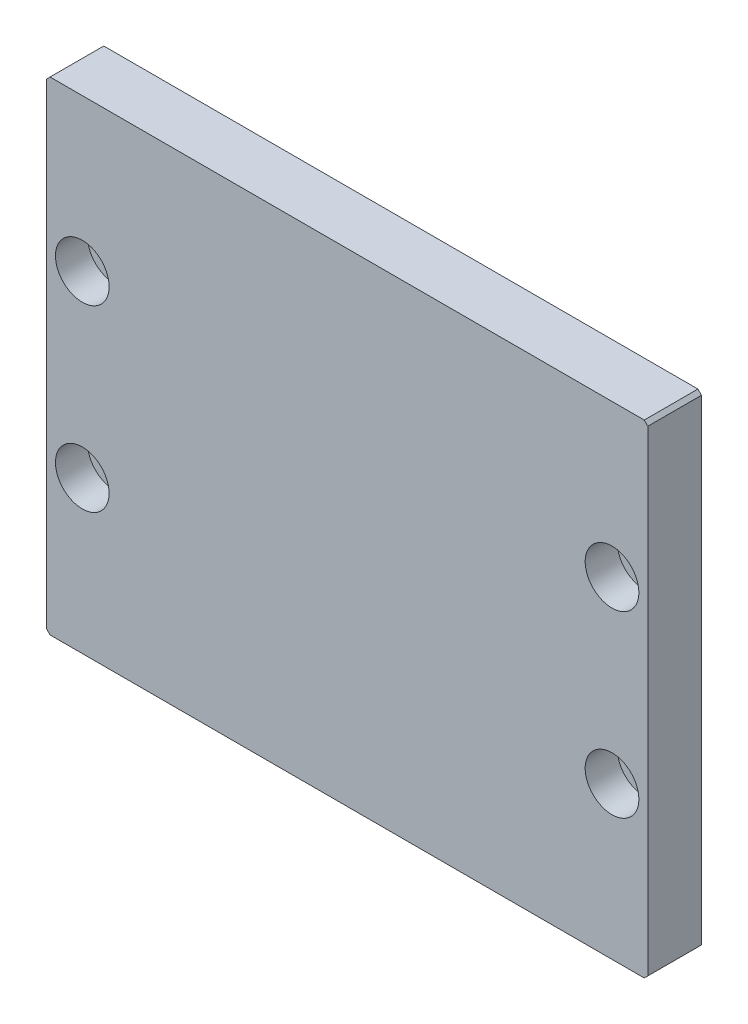
from build123d import *

# Parameters (mm, degrees)
SKETCH1_W                                            = 168
SKETCH1_H                                            = 135
BOSS_EXTRUDE1_DEPTH                                  = 15
HOLE_SIZE_PER_SOCKET_HEAD_CAP_SCREW_TYPE_D           = 9
HOLE_SIZE_PER_SOCKET_HEAD_CAP_SCREW_TYPE_CBORE_D     = 15
HOLE_SIZE_PER_SOCKET_HEAD_CAP_SCREW_TYPE_CBORE_DEPTH = 9
CHAMFER1_SIZE                                        = 1


with BuildPart() as part:
    # Sketch1 → Boss-Extrude1 (new body)
    with BuildSketch(Plane.XY):
        Rectangle(SKETCH1_W, SKETCH1_H)
    extrude(amount=BOSS_EXTRUDE1_DEPTH)

    # Hole size per socket head cap screw type1 (through all)
    with Locations(Plane.XY.offset(15)):
        with Locations((-74, 25), (-74, -25), (74, -25), (74, 25)):
            CounterBoreHole(HOLE_SIZE_PER_SOCKET_HEAD_CAP_SCREW_TYPE_D / 2, HOLE_SIZE_PER_SOCKET_HEAD_CAP_SCREW_TYPE_CBORE_D / 2, HOLE_SIZE_PER_SOCKET_HEAD_CAP_SCREW_TYPE_CBORE_DEPTH)

    # Chamfer1
    chamfer1_edges = [part.edges().sort_by_distance(p)[0] for p in [
        (84, -67.5, 7.5),
        (-84, -67.5, 7.5),
        (-84, 67.5, 7.5),
        (84, 67.5, 7.5),
    ]]
    chamfer(chamfer1_edges, length=CHAMFER1_SIZE)


solid = part.part
